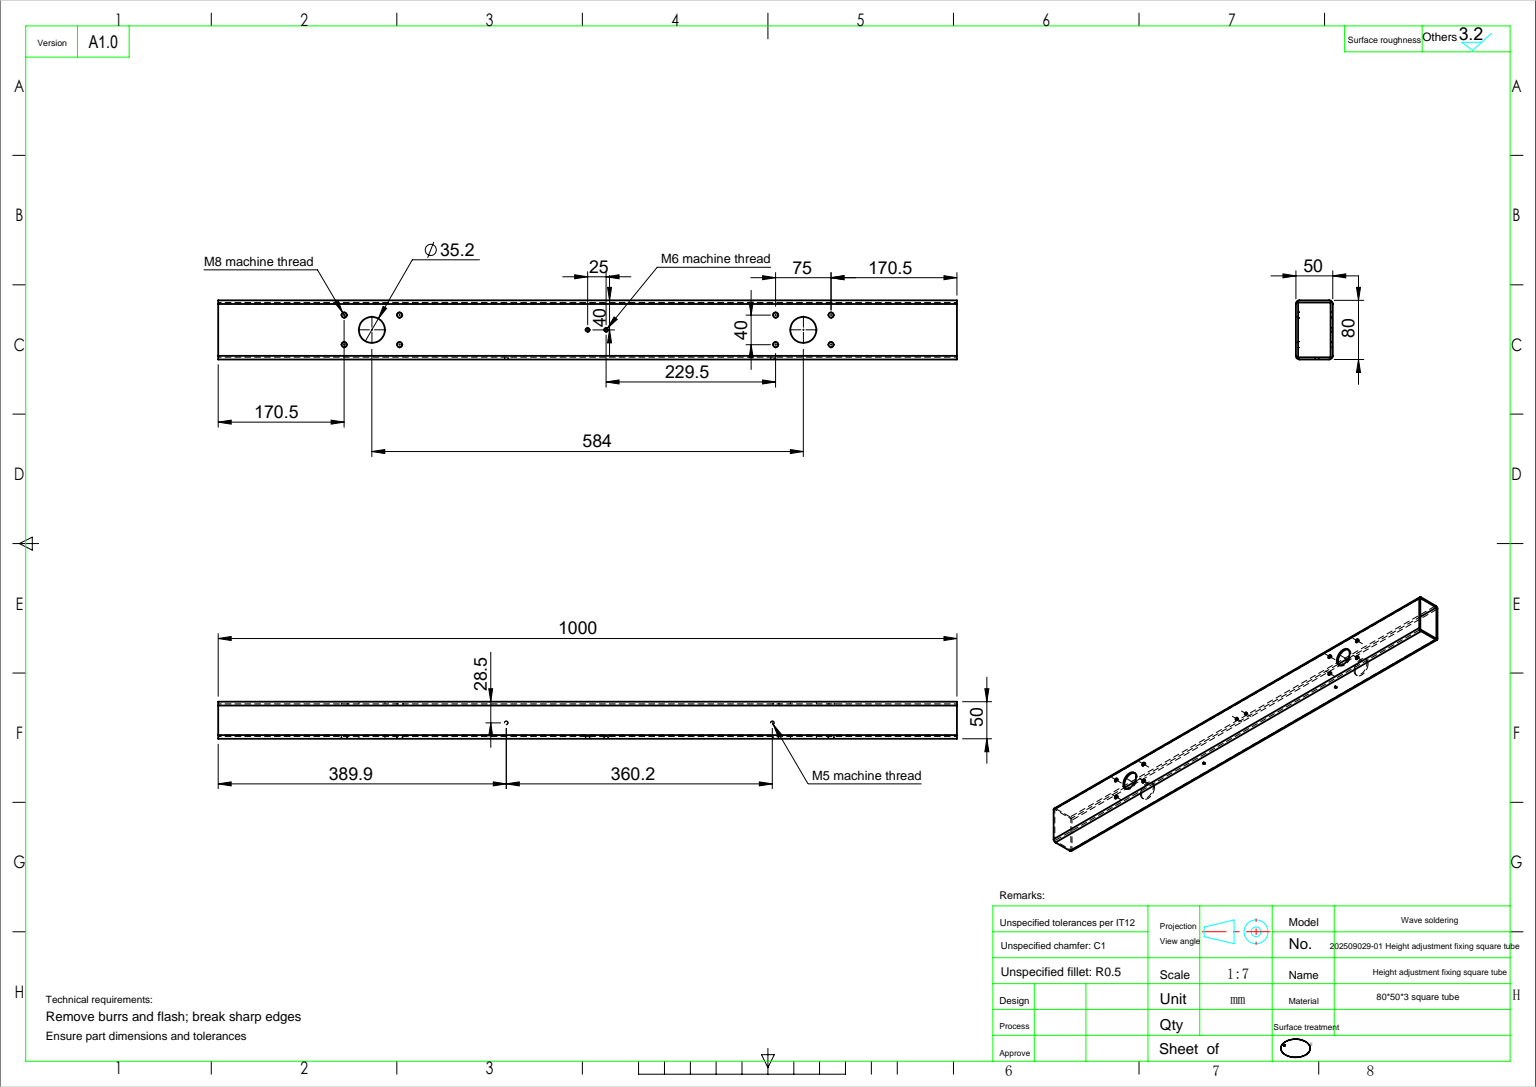
from build123d import *

# Parameters (mm, degrees)
SKETCH_1_W          = 1000
SKETCH_1_H          = 80
EXTRUDE_1_DEPTH     = 50
SHELL_1_T           = -3
FILLET_1_R          = 5
SKETCH_3_R          = 17.6
CUT_EXTRUDE_2_DEPTH = 505.083326445
SKETCH_4_R          = 3.4
CUT_EXTRUDE_3_DEPTH = 10
SKETCH_5_R          = 2.5
CUT_EXTRUDE_4_DEPTH = 10
SKETCH_6_R          = 2.1
CUT_EXTRUDE_5_DEPTH = 10


with BuildPart() as part:
    # 草图1 → 凸台-拉伸1 (new body)
    with BuildSketch(Plane.XY):
        Rectangle(SKETCH_1_W, SKETCH_1_H)
    extrude(amount=EXTRUDE_1_DEPTH)

    # 抽壳1
    shell_1_openings = [part.faces().sort_by_distance(p)[0] for p in [
        (-500, 0, 25),
        (500, 0, 25),
    ]]
    offset(amount=SHELL_1_T, openings=shell_1_openings, kind=Kind.INTERSECTION)

    # 圆角1
    fillet_1_edges = [part.edges().sort_by_distance(p)[0] for p in [
        (0, -40, 50),
        (0, -40, 0),
        (0, 40, 0),
        (0, 40, 50),
    ]]
    fillet(fillet_1_edges, radius=FILLET_1_R)

    # 草图3 → 切除-拉伸2 (cut, through all)
    with BuildSketch(Plane(origin=(0, 0, 0), x_dir=(-1, 0, 0), z_dir=(0, 0, -1))):
        with Locations((-292, 0)):
            Circle(SKETCH_3_R)
        with Locations((292, 0)):
            Circle(SKETCH_3_R)
    extrude(amount=-CUT_EXTRUDE_2_DEPTH, mode=Mode.SUBTRACT)

    # 草图4 → 切除-拉伸3 (cut)
    with BuildSketch(Plane(origin=(0, 0, 0), x_dir=(-1, 0, 0), z_dir=(0, 0, -1))):
        with Locations((-329.5, 20)):
            Circle(SKETCH_4_R)
        with Locations((-329.5, -20)):
            Circle(SKETCH_4_R)
        with Locations((-254.5, 20)):
            Circle(SKETCH_4_R)
        with Locations((-254.5, -20)):
            Circle(SKETCH_4_R)
        with Locations((254.5, 20)):
            Circle(SKETCH_4_R)
        with Locations((254.5, -20)):
            Circle(SKETCH_4_R)
        with Locations((329.5, 20)):
            Circle(SKETCH_4_R)
        with Locations((329.5, -20)):
            Circle(SKETCH_4_R)
    extrude(amount=-CUT_EXTRUDE_3_DEPTH, mode=Mode.SUBTRACT)

    # 草图5 → 切除-拉伸4 (cut)
    with BuildSketch(Plane(origin=(0, 0, 0), x_dir=(-1, 0, 0), z_dir=(0, 0, -1))):
        Circle(SKETCH_5_R)
        with Locations((25, 0)):
            Circle(SKETCH_5_R)
    extrude(amount=-CUT_EXTRUDE_4_DEPTH, mode=Mode.SUBTRACT)

    # 草图6 → 切除-拉伸5 (cut)
    with BuildSketch(Plane.XZ.offset(40)):
        with Locations(Location((110.1, 21.5, 0), (0, 0, 270))):
            Circle(SKETCH_6_R)
        with Locations(Location((-250.1, 21.5, 0), (0, 0, 270))):
            Circle(SKETCH_6_R)
    extrude(amount=-CUT_EXTRUDE_5_DEPTH, mode=Mode.SUBTRACT)


solid = part.part
